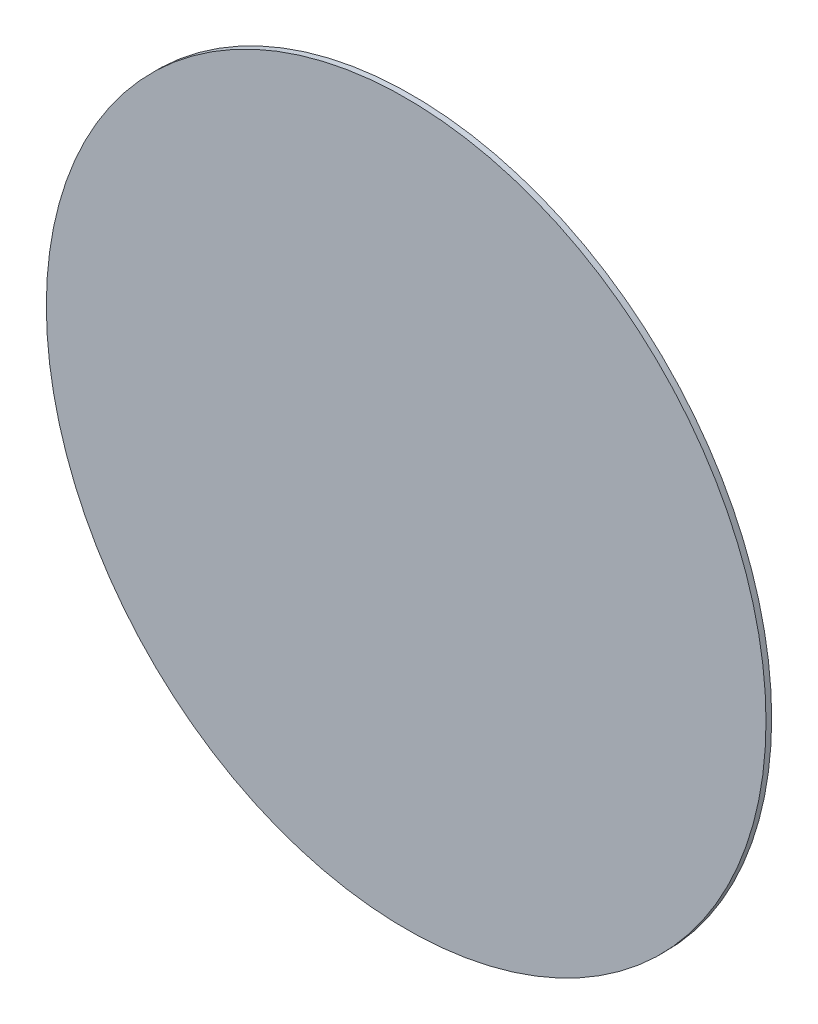
SolidWorks part; units mm, degrees
ref_plane "Front" through (0, 0, 0) normal (0, 0, 1) x (1, 0, 0)
ref_plane "Top" through (0, 0, 0) normal (0, 1, 0) x (1, 0, 0)
ref_plane "Right" through (0, 0, 0) normal (1, 0, 0) x (0, 0, -1)
sketch "Sketch1" plane through (0, 0, 0) normal (0, 0, 1) x (1, 0, 0)
  circle A0 centre (0, 0) radius 127
extrude "Boss-Extrude1" add sketch "Sketch1" along normal up to surface (2 mm away) contours A0
